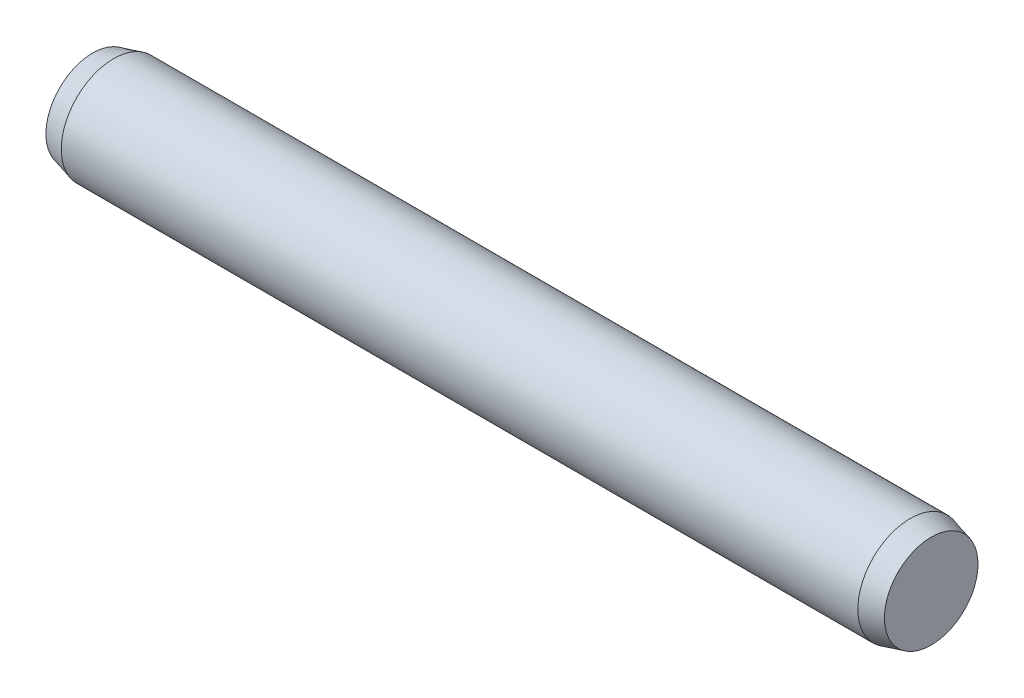
from build123d import *


with BuildPart() as part:
    # Dimensioned Sketch → Base-Revolve (revolve)
    with BuildSketch(Plane.XY, mode=Mode.PRIVATE) as base_revolve_sk:
        Polygon((0, 0), (80, 0), (80, 4.464101615), (78, 5), (2, 5), (0, 4.464101615), align=None)
    revolve(base_revolve_sk.sketch.rotate(Axis((0, 0, 0), (-1, 0, 0)), 90), axis=Axis((0, 0, 0), (-1, 0, 0)))


solid = part.part
